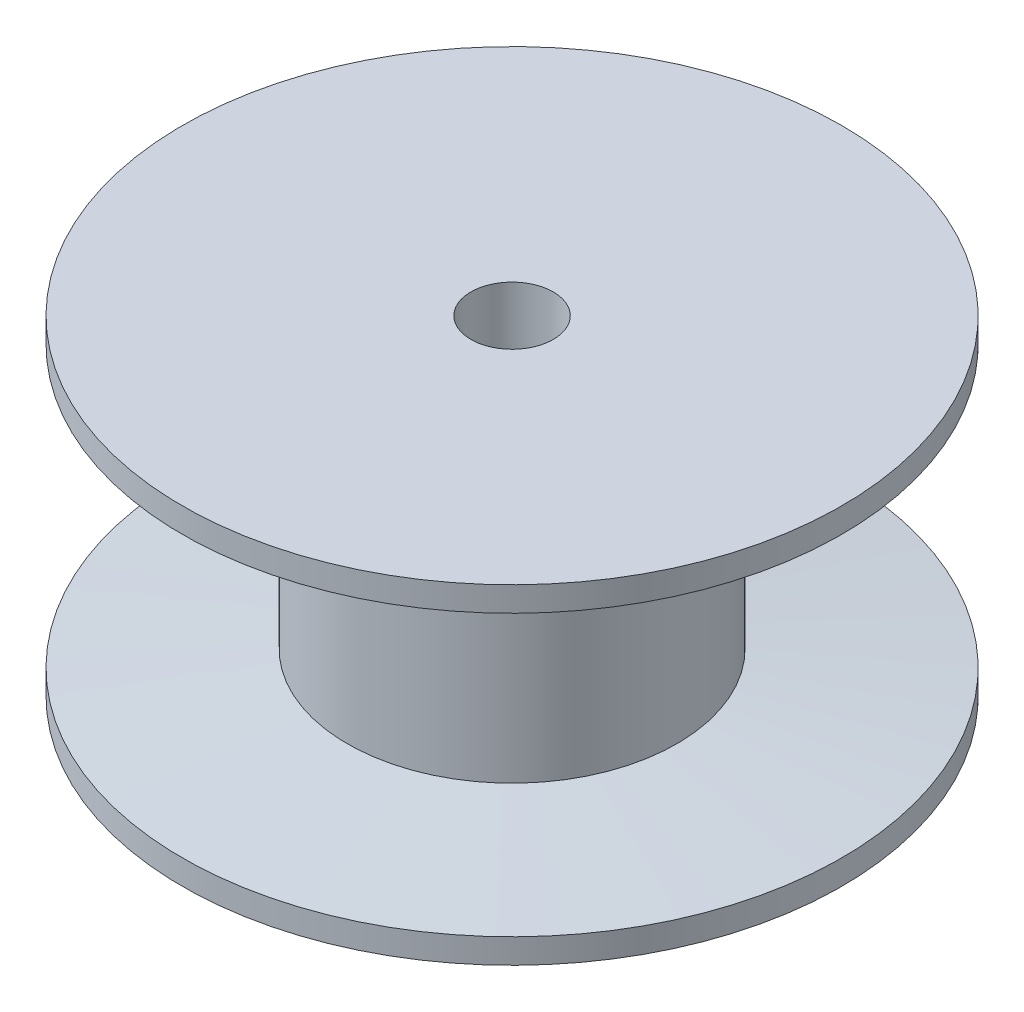
from build123d import *


with BuildPart() as part:
    # 草图1 → 旋转1 (revolve)
    with BuildSketch(Plane(origin=(0, 0, 0), x_dir=(0, 0, -1), z_dir=(1, 0, 0))):
        Polygon((5, 0), (40, 0), (40, 3), (20, 5), (20, 35), (40, 37), (40, 40), (5, 40), align=None)
    revolve(axis=Axis((0, 0, 0), (0, 1, 0)))


solid = part.part
